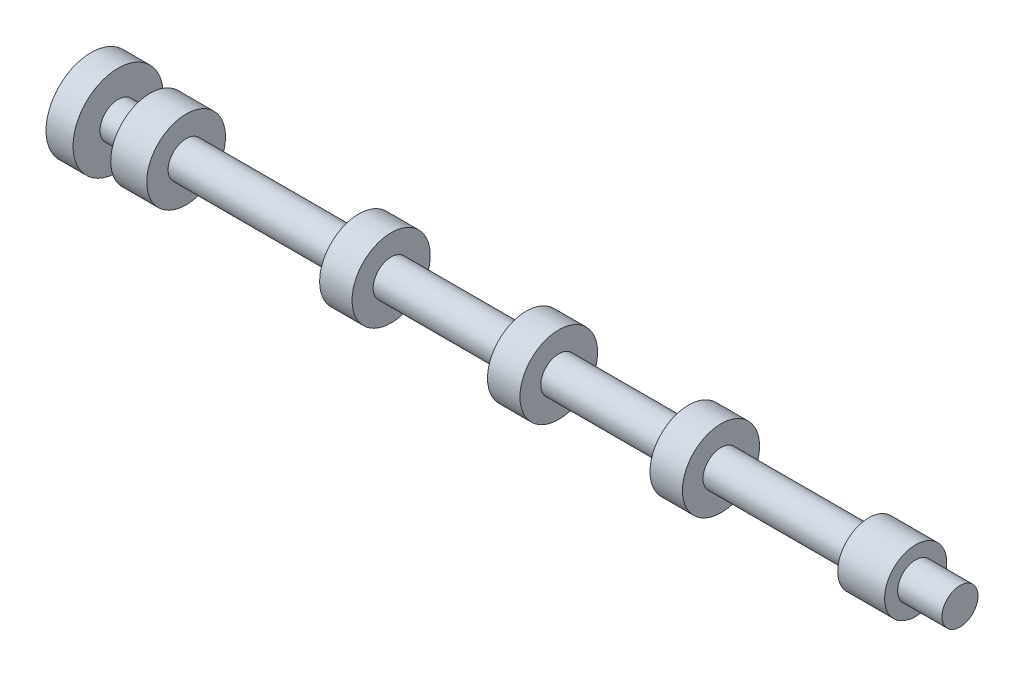
SolidWorks part; units mm, degrees
ref_plane "Front Plane" through (0, 0, 0) normal (0, 0, 1) x (1, 0, 0)
ref_plane "Top Plane" through (0, 0, 0) normal (0, 1, 0) x (1, 0, 0)
ref_plane "Right Plane" through (0, 0, 0) normal (1, 0, 0) x (0, 0, -1)
sketch "Sketch1" plane through (0, 0, 0) normal (0, 0, 1) x (1, 0, 0)
  line L0 (-2966.6704, 0) -> (-2484.5704, 0)
  line L1 (-2966.6704, 0) -> (-2966.6704, 25)
  line L2 (-2966.6704, 25) -> (-2951.6704, 25)
  line L29 (-2951.6704, 25) -> (-2951.6704, 10)
  line L30 (-2951.6704, 10) -> (-2933.92, 10)
  line L31 (-2933.92, 10) -> (-2933.92, 21.85)
  line L32 (-2933.92, 21.85) -> (-2913.92, 21.85)
  line L33 (-2913.92, 21.85) -> (-2913.92, 10)
  line L34 (-2913.92, 10) -> (-2818.1701, 10)
  line L35 (-2818.1701, 10) -> (-2818.1701, 21.7)
  line L36 (-2818.1701, 21.7) -> (-2800.1701, 21.7)
  line L37 (-2800.1701, 21.7) -> (-2800.1701, 10)
  line L38 (-2800.1701, 10) -> (-2725.1703, 10)
  line L39 (-2725.1703, 10) -> (-2725.1703, 21.55)
  line L40 (-2725.1703, 21.55) -> (-2707.1703, 21.55)
  line L41 (-2707.1703, 21.55) -> (-2707.1703, 10)
  line L42 (-2707.1703, 10) -> (-2635.1704, 10)
  line L43 (-2635.1704, 10) -> (-2635.1704, 21.4)
  line L44 (-2635.1704, 21.4) -> (-2617.1704, 21.4)
  line L45 (-2617.1704, 21.4) -> (-2617.1704, 10)
  line L46 (-2617.1704, 10) -> (-2535.1704, 10)
  line L47 (-2535.1704, 10) -> (-2535.1704, 17.25)
  line L48 (-2535.1704, 17.25) -> (-2509.1704, 17.25)
  line L49 (-2509.1704, 17.25) -> (-2509.1704, 10)
  line L50 (-2509.1704, 10) -> (-2484.5704, 10)
  line L51 (-2484.5704, 10) -> (-2484.5704, 0)
  point P16 (-2522.1704, 17.25)
  point P28 (-2626.1704, 21.4)
  point P29 (-2716.1703, 21.55)
  point P30 (-2809.1701, 21.7)
  point P31 (-2923.92, 21.85)
  dimension "D1" = 482.1
  dimension "D2" = 25
  dimension "D3" = 26
  dimension "D4" = 18
  dimension "D5" = 18
  dimension "D6" = 18
  dimension "D7" = 20
  dimension "D9" = 104
  dimension "D10" = 90
  dimension "D11" = 93
  dimension "D12" = 114.75
  dimension "D13" = 15
  dimension "D14" = 21.85
  dimension "D15" = 21.7
  dimension "D16" = 21.55
  dimension "D17" = 21.4
  dimension "D18" = 17.25
  dimension "D19" = 10
  dimension "D20" = 10
  dimension "D21" = 10
  dimension "D22" = 10
  dimension "D23" = 10
  dimension "D24" = 10
revolve "Revolve1" add sketch "Sketch1" angle 360 about L0
